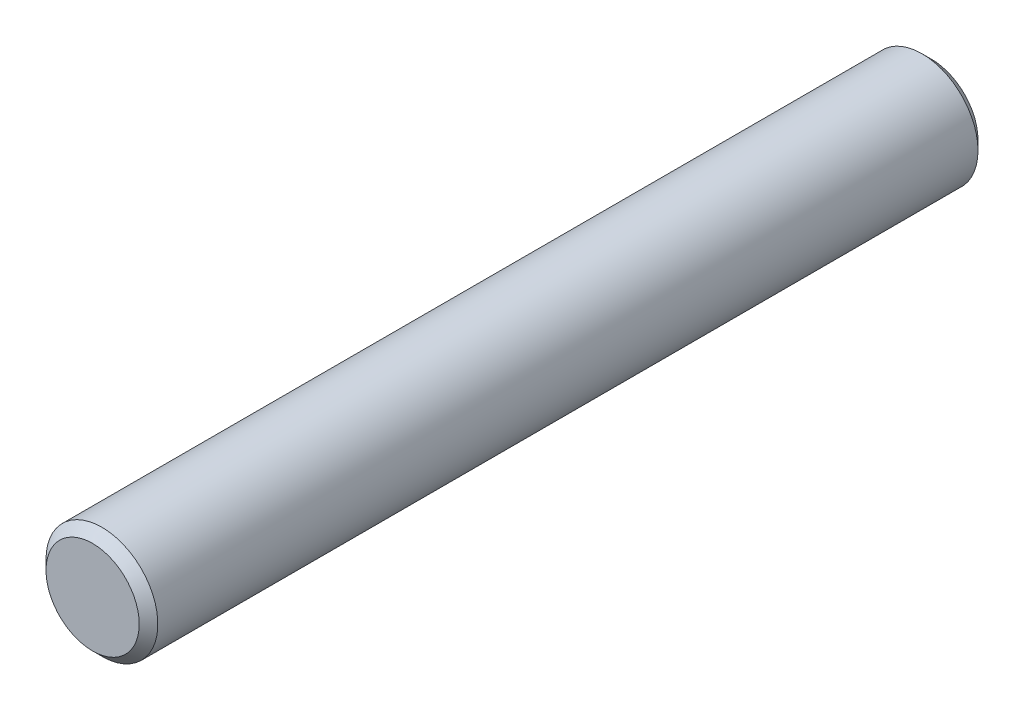
from build123d import *

# Parameters (mm, degrees)
SKETCH_1_R             = 3
EXTRUDE_1_DEPTH        = 45
HOLE_WIZARD_M3_1_D     = 2.5
HOLE_WIZARD_M3_1_DEPTH = 7.5
HOLE_WIZARD_M3_1_TIP   = 0.751075774
CHAMFER_1_SIZE         = 0.5


with BuildPart() as part:
    # 草图1 → 凸台-拉伸1 (new body)
    with BuildSketch(Plane.XY):
        with Locations(Location((0, 0, 0), (0, 0, 180))):
            Circle(SKETCH_1_R)
    extrude(amount=EXTRUDE_1_DEPTH)

    # M3 螺纹孔1
    with Locations(Plane(origin=(0, 0, 0), x_dir=(-1, 0, 0), z_dir=(0, 0, -1))):
        with Locations((0, 0)):
            Hole(HOLE_WIZARD_M3_1_D / 2, depth=HOLE_WIZARD_M3_1_DEPTH)
            with Locations((0, 0, -(HOLE_WIZARD_M3_1_DEPTH + HOLE_WIZARD_M3_1_TIP / 2))):  # 118° drill point
                Cone(0, HOLE_WIZARD_M3_1_D / 2, HOLE_WIZARD_M3_1_TIP, mode=Mode.SUBTRACT)

    # 倒角1
    chamfer_1_edges = [part.edges().sort_by_distance(p)[0] for p in [
        (3, 0, 0),
        (3, 0, 45),
    ]]
    chamfer(chamfer_1_edges, length=CHAMFER_1_SIZE)


solid = part.part
